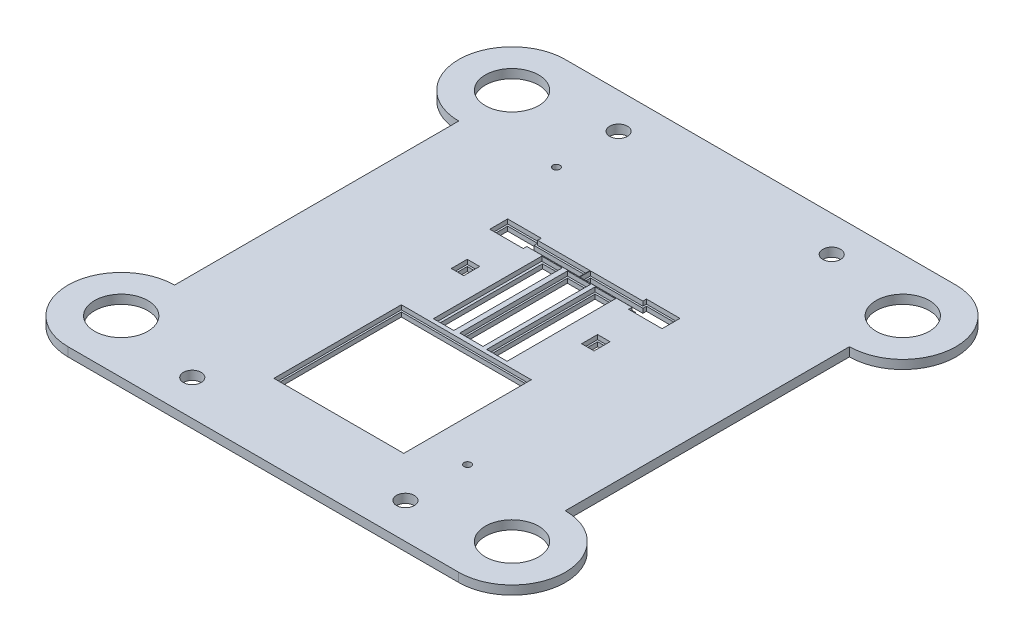
from build123d import *

# Parameters (mm, degrees)
SKETCH2_R           = 15
BOSS_EXTRUDE1_DEPTH = 5
SKETCH3_W           = 73.144376366
SKETCH3_H           = 71.78
SKETCH3_W_2         = 7
SKETCH3_H_2         = 9
SKETCH3_W_3         = 11.5
SKETCH3_H_3         = 61
SKETCH3_W_4         = 13.06
SKETCH3_H_4         = 60.56
CUT_EXTRUDE1_DEPTH  = 2.5
SKETCH4_W           = 11.06
SKETCH4_H           = 58.56
SKETCH4_W_2         = 9.088350763
SKETCH4_H_2         = 59
SKETCH4_W_3         = 5
SKETCH4_H_3         = 7
SKETCH4_W_4         = 71.144376366
SKETCH4_H_4         = 69.78
CUT_EXTRUDE3_DEPTH  = 5
SKETCH5_R           = 5
CUT_EXTRUDE4_DEPTH  = 179.115131306
BOSS_EXTRUDE2_DEPTH = 5
SKETCH_2_R          = 15
CUT_EXTRUDE2_DEPTH  = 5
SKETCH_3_R          = 2
CUT_EXTRUDE_3_DEPTH = 221.283907719


with BuildPart() as part:
    # Sketch2 → Boss-Extrude1 (new body)
    with BuildSketch(Plane(origin=(0, 0, 0), x_dir=(1, 0, 0), z_dir=(0, 1, 0))):
        with BuildLine():
            Line((-80, -140), (110, -140))
            Line((110, -140), (110, 140))
            Line((110, 140), (-80, 140))
            ThreePointArc((-80, 140), (-110, 110), (-80, 80))
            Line((-80, 80), (-80, -80))
            ThreePointArc((-80, -80), (-110, -110), (-80, -140))
        make_face()
        with Locations(Location((-80, 110, 0), (0, 0, 270))):
            Circle(SKETCH2_R, mode=Mode.SUBTRACT)
        with Locations(Location((-80, -110, 0), (0, 0, 270))):
            Circle(SKETCH2_R, mode=Mode.SUBTRACT)
    extrude(amount=BOSS_EXTRUDE1_DEPTH)

    # Sketch3 → Cut-Extrude1 (cut)
    with BuildSketch(Plane(origin=(0, 5, 0), x_dir=(1, 0, 0), z_dir=(0, 1, 0))):
        Polygon((0.37, 46.06), (0.37, 44.06), (29.86, 44.06), (29.86, 38), (0.37, 38), (0.37, 36), (-18.5, 36), (-18.5, 46.06), align=None)
        with Locations((30, -61.61)):
            Rectangle(SKETCH3_W, SKETCH3_H)
        with Locations((-6.69, 10.5)):
            Rectangle(SKETCH3_W_2, SKETCH3_H_2)
        with Locations((66.69, 10.5)):
            Rectangle(SKETCH3_W_2, SKETCH3_H_2)
        with Locations((45, 7)):
            Rectangle(SKETCH3_W_3, SKETCH3_H_3)
        with Locations((30.22, 7.22)):
            Rectangle(SKETCH3_W_4, SKETCH3_H_4)
        with Locations((15, 7)):
            Rectangle(SKETCH3_W_3, SKETCH3_H_3)
        Polygon((78.5, 46.06), (59.63, 46.06), (59.63, 44.06), (30.14, 44.06), (30.14, 38), (59.63, 38), (59.63, 36), (78.5, 36), align=None)
    extrude(amount=-CUT_EXTRUDE1_DEPTH, mode=Mode.SUBTRACT)

    # Sketch4 → Cut-Extrude3 (cut)
    with BuildSketch(Plane(origin=(0, 5, 0), x_dir=(1, 0, 0), z_dir=(0, 1, 0))):
        with Locations((30.22, 7.22)):
            Rectangle(SKETCH4_W, SKETCH4_H)
        Polygon((-0.601649237, 45.06), (-0.601649237, 43.06), (28.888350763, 43.06), (28.888350763, 39), (-0.601649237, 39), (-0.601649237, 37), (-17.471649237, 37), (-17.471649237, 45.06), align=None)
        Polygon((31.14, 43.06), (31.14, 39), (60.63, 39), (60.63, 37), (77.5, 37), (77.5, 45.06), (60.63, 45.06), (60.63, 43.06), align=None)
        with Locations((44.794175381, 7)):
            Rectangle(SKETCH4_W_2, SKETCH4_H_2)
        with Locations((66.69, 10.5)):
            Rectangle(SKETCH4_W_3, SKETCH4_H_3)
        with Locations((30, -61.61)):
            Rectangle(SKETCH4_W_4, SKETCH4_H_4)
        with Locations((15.234175382, 7)):
            Rectangle(SKETCH4_W_2, SKETCH4_H_2)
        with Locations((-6.661649237, 10.5)):
            Rectangle(SKETCH4_W_3, SKETCH4_H_3)
    extrude(amount=-CUT_EXTRUDE3_DEPTH, mode=Mode.SUBTRACT)

    # Sketch5 → Cut-Extrude4 (cut, through all)
    with BuildSketch(Plane(origin=(0, 5, 0), x_dir=(1, 0, 0), z_dir=(0, 1, 0))):
        with Locations(Location((-30, 120, 0), (0, 0, 270))):
            Circle(SKETCH5_R)
        with Locations(Location((90, 120, 0), (0, 0, 270))):
            Circle(SKETCH5_R)
        with Locations(Location((90, -120, 0), (0, 0, 270))):
            Circle(SKETCH5_R)
        with Locations(Location((-30, -120, 0), (0, 0, 270))):
            Circle(SKETCH5_R)
    extrude(amount=-CUT_EXTRUDE4_DEPTH, mode=Mode.SUBTRACT)

    # Sketch1 → Boss-Extrude2 (add)
    with BuildSketch(Plane(origin=(0, 5, 0), x_dir=(1, 0, 0), z_dir=(0, 1, 0))):
        with BuildLine():
            Line((108.024540476, 140), (140, 140))
            ThreePointArc((140, 140), (170, 110), (140, 80))
            Line((140, 80), (140, -80))
            ThreePointArc((140, -80), (170, -110), (140, -140))
            Line((140, -140), (108.024540476, -140))
            Line((108.024540476, -140), (108.024540476, 140))
        make_face()
    extrude(amount=-BOSS_EXTRUDE2_DEPTH)

    # 草图2 → Cut-Extrude2 (cut)
    with BuildSketch(Plane(origin=(0, 5, 0), x_dir=(1, 0, 0), z_dir=(0, 1, 0))):
        with Locations(Location((140, 110, 0), (0, 0, 270))):
            Circle(SKETCH_2_R)
        with Locations(Location((140, -110, 0), (0, 0, 270))):
            Circle(SKETCH_2_R)
    extrude(amount=-CUT_EXTRUDE2_DEPTH, mode=Mode.SUBTRACT)

    # 草图3 → 切除-拉伸3 (cut, through all)
    with BuildSketch(Plane(origin=(0, 5, 0), x_dir=(1, 0, 0), z_dir=(0, 1, 0))):
        with Locations(Location((-30, 85, 0), (0, 0, 270))):
            Circle(SKETCH_3_R)
        with Locations(Location((90, -85, 0), (0, 0, 270))):
            Circle(SKETCH_3_R)
    extrude(amount=-CUT_EXTRUDE_3_DEPTH, mode=Mode.SUBTRACT)


solid = part.part
